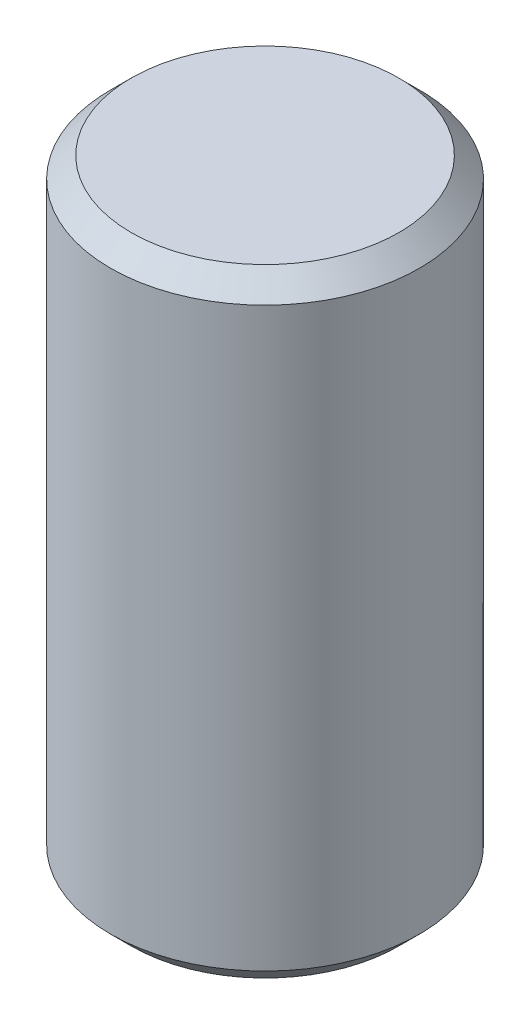
from build123d import *

# Parameters (mm, degrees)
SKETCH1_R           = 1.5
BOSS_EXTRUDE1_DEPTH = 6
CHAMFER1_SIZE       = 0.2


with BuildPart() as part:
    # Sketch1 → Boss-Extrude1 (new body)
    with BuildSketch(Plane(origin=(0, 0, 0), x_dir=(1, 0, 0), z_dir=(0, 1, 0))):
        with Locations(Location((0, 0, 0), (0, 0, 270))):
            Circle(SKETCH1_R)
    extrude(amount=BOSS_EXTRUDE1_DEPTH)

    # Chamfer1
    chamfer1_edges = [part.edges().sort_by_distance(p)[0] for p in [
        (0, 0, -1.5),
        (0, 6, -1.5),
    ]]
    chamfer(chamfer1_edges, length=CHAMFER1_SIZE)


solid = part.part
